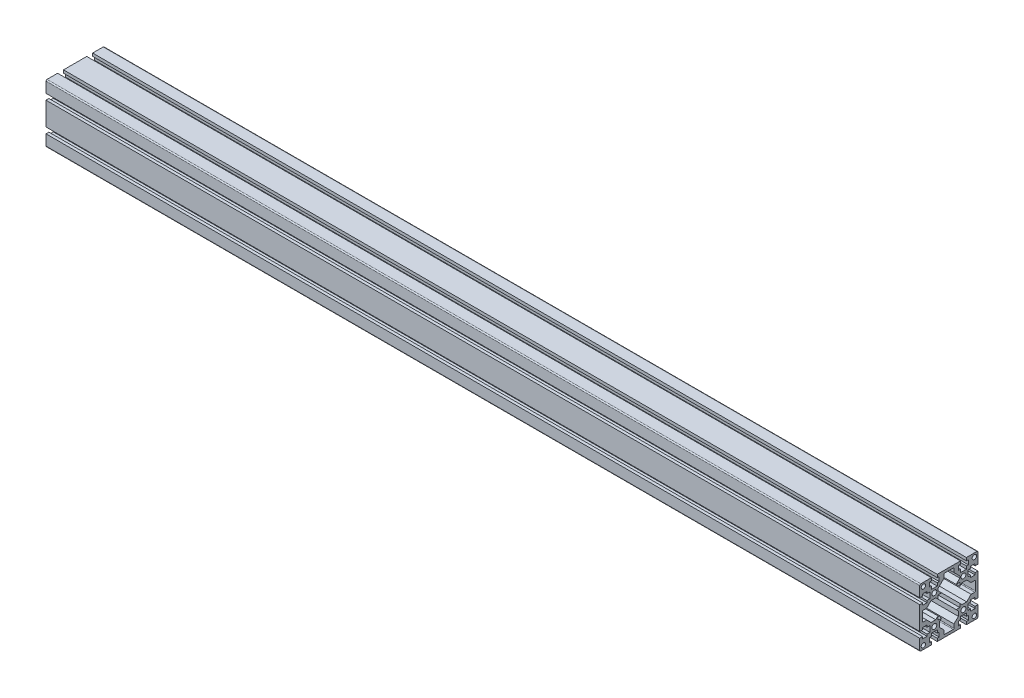
SolidWorks part; units mm, degrees
ref_plane "Front Plane" through (0, 0, 0) normal (0, 0, 1) x (1, 0, 0)
ref_plane "Top Plane" through (0, 0, 0) normal (0, 1, 0) x (1, 0, 0)
ref_plane "Right Plane" through (0, 0, 0) normal (1, 0, 0) x (0, 0, -1)
sketch "草图1" plane through (0, 0, 0) normal (0, 0, 1) x (1, 0, 0)
  line L0 (-530.3448, 0) -> (669.6552, 0)
  dimension "D1" = 1200
other "Aluminum profile 80 X 80G X R1.5(1)"
ref_plane "Plane2" through (-530.3448, 0, 0) normal (1, 0, 0) x (0, 1, 0)
sketch "Sketch1" plane through (-530.3448, 0, 0) normal (1, 0, 0) x (0, 1, 0)
  line L0 (0, 40) -> (0, 0) construction
  line L1 (0, 0) -> (40, 0) construction
  line L2 (-24.05, 40) -> (-24.05, 36)
  line L3 (-38.5, 40) -> (-24.05, 40)
  line L4 (-40, 38.5) -> (-40, 24.05)
  line L5 (-38.5, -40) -> (-24.05, -40)
  line L6 (40, 38.5) -> (40, 24.05)
  line L7 (-24.05, 36) -> (-26.75, 36)
  line L8 (-26.75, 36) -> (-26.75, 30)
  line L9 (-26.75, 30) -> (-24.05, 30)
  line L10 (-24.05, 30) -> (-24.05, 26)
  line L11 (-24.05, 26) -> (-15.95, 26)
  line L12 (-15.95, 26) -> (-15.95, 30)
  line L13 (-15.95, 30) -> (-13.25, 30)
  line L14 (-13.25, 30) -> (-13.25, 36)
  line L15 (-13.25, 36) -> (-15.95, 36)
  line L16 (-15.95, 36) -> (-15.95, 40)
  line L17 (-40, 15.95) -> (-36, 15.95)
  line L18 (-36, 15.95) -> (-36, 13.25)
  line L19 (-15.95, 40) -> (15.95, 40)
  line L20 (-20, 20) -> (-20, 40) construction
  line L21 (20, 20) -> (20, 40) construction
  line L22 (15.95, 36) -> (15.95, 40)
  line L23 (13.25, 36) -> (15.95, 36)
  line L24 (13.25, 30) -> (13.25, 36)
  line L25 (15.95, 30) -> (13.25, 30)
  line L26 (-36, 13.25) -> (-30, 13.25)
  line L27 (-30, 13.25) -> (-30, 15.95)
  line L28 (-26, 15.95) -> (-26, 24.05)
  line L29 (-26, 24.05) -> (-30, 24.05)
  line L30 (-30, 24.05) -> (-30, 26.75)
  line L31 (-30, 26.75) -> (-36, 26.75)
  line L32 (-36, 26.75) -> (-36, 24.05)
  line L33 (-36, 24.05) -> (-40, 24.05)
  line L34 (-30, 15.95) -> (-26, 15.95)
  line L35 (15.95, 26) -> (15.95, 30)
  line L36 (24.05, 26) -> (15.95, 26)
  line L37 (24.05, 30) -> (24.05, 26)
  line L38 (26.75, 30) -> (24.05, 30)
  line L39 (26.75, 36) -> (26.75, 30)
  line L40 (24.05, 36) -> (26.75, 36)
  line L41 (24.05, 40) -> (24.05, 36)
  line L42 (24.05, -40) -> (24.05, -36)
  line L43 (24.05, -36) -> (26.75, -36)
  line L44 (26.75, -36) -> (26.75, -30)
  line L45 (26.75, -30) -> (24.05, -30)
  line L46 (24.05, -30) -> (24.05, -26)
  line L47 (24.05, -26) -> (15.95, -26)
  line L48 (15.95, -26) -> (15.95, -30)
  line L49 (15.95, -30) -> (13.25, -30)
  line L50 (13.25, -30) -> (13.25, -36)
  line L51 (13.25, -36) -> (15.95, -36)
  line L52 (15.95, -36) -> (15.95, -40)
  line L53 (-15.95, -36) -> (-15.95, -40)
  line L54 (-13.25, -36) -> (-15.95, -36)
  line L55 (-13.25, -30) -> (-13.25, -36)
  line L56 (-15.95, -30) -> (-13.25, -30)
  line L57 (-15.95, -26) -> (-15.95, -30)
  line L58 (-24.05, -26) -> (-15.95, -26)
  line L59 (-24.05, -30) -> (-24.05, -26)
  line L60 (-26.75, -30) -> (-24.05, -30)
  line L61 (-26.75, -36) -> (-26.75, -30)
  line L62 (-24.05, -36) -> (-26.75, -36)
  line L63 (-24.05, -40) -> (-24.05, -36)
  line L64 (-30, -15.95) -> (-26, -15.95)
  line L65 (-36, -26.75) -> (-36, -24.05)
  line L66 (-30, -26.75) -> (-36, -26.75)
  line L67 (-30, -24.05) -> (-30, -26.75)
  line L68 (-26, -24.05) -> (-30, -24.05)
  line L69 (-26, -15.95) -> (-26, -24.05)
  line L70 (-30, -13.25) -> (-30, -15.95)
  line L71 (-36, -13.25) -> (-30, -13.25)
  line L72 (-36, -15.95) -> (-36, -13.25)
  line L73 (36, 24.05) -> (40, 24.05)
  line L74 (40, 15.95) -> (36, 15.95)
  line L75 (36, -15.95) -> (36, -13.25)
  line L76 (36, -13.25) -> (30, -13.25)
  line L77 (30, -13.25) -> (30, -15.95)
  line L78 (26, -15.95) -> (26, -24.05)
  line L79 (26, -24.05) -> (30, -24.05)
  line L80 (30, -24.05) -> (30, -26.75)
  line L81 (30, -26.75) -> (36, -26.75)
  line L82 (36, -26.75) -> (36, -24.05)
  line L83 (30, -15.95) -> (26, -15.95)
  line L84 (30, 15.95) -> (26, 15.95)
  line L85 (36, 26.75) -> (36, 24.05)
  line L86 (30, 26.75) -> (36, 26.75)
  line L87 (30, 24.05) -> (30, 26.75)
  line L88 (26, 24.05) -> (30, 24.05)
  line L89 (26, 15.95) -> (26, 24.05)
  line L90 (30, 13.25) -> (30, 15.95)
  line L91 (36, 13.25) -> (30, 13.25)
  line L92 (36, 15.95) -> (36, 13.25)
  line L93 (-36, -15.95) -> (-40, -15.95)
  line L94 (-36, -24.05) -> (-40, -24.05)
  line L95 (36, -15.95) -> (40, -15.95)
  line L96 (36, -24.05) -> (40, -24.05)
  line L97 (-13, 18) -> (-10, 15)
  line L98 (-15, 15) -> (-10, 15)
  line L99 (-15, 15) -> (-15, 10)
  line L100 (-15, -15) -> (-10, -15)
  line L101 (15, 15) -> (15, 10)
  line L102 (-18, 13) -> (-15, 10)
  line L104 (13, 18) -> (10, 15)
  line L105 (13, -18) -> (10, -15)
  line L106 (20, -15) -> (15, -10)
  line L107 (-18, -13) -> (-15, -10)
  line L108 (-13, -18) -> (-10, -15)
  line L109 (15, -10) -> (15, -15)
  line L110 (10, 15) -> (15, 15)
  line L111 (-15, -10) -> (-15, -15)
  line L112 (10, -15) -> (15, -15)
  line L113 (15, 10) -> (20, 15)
  line L235 (24.05, 40) -> (38.5, 40)
  line L249 (-40, 15.95) -> (-40, -15.95)
  line L250 (-20, 20) -> (-26, 20) construction
  line L264 (40, 15.95) -> (40, -15.95)
  line L265 (-13, 24.5) -> (-7, 30.5)
  line L266 (-7, 30.5) -> (-7, 35.5)
  line L267 (7, 35.5) -> (7, 30.5)
  line L268 (7, 30.5) -> (13, 24.5)
  line L269 (-6, -36.5) -> (6, -36.5)
  line L270 (-13, 24.5) -> (-13, 18)
  line L271 (-35.5, 7) -> (-30.5, 7)
  line L272 (-30.5, 7) -> (-24.5, 13)
  line L273 (-24.5, 13) -> (-18, 13)
  line L274 (13, 24.5) -> (13, 18)
  line L275 (-15.95, -40) -> (15.95, -40)
  line L276 (35.5, 7) -> (30.5, 7)
  line L277 (30.5, 7) -> (22.5, 15)
  line L278 (24.05, -40) -> (38.5, -40)
  line L279 (20, 15) -> (22.5, 15)
  line L333 (-13, -24.5) -> (-13, -18)
  line L336 (-13, -24.5) -> (-7, -30.5)
  line L385 (-7, -30.5) -> (-7, -35.5)
  line L386 (-36.5, 6) -> (-36.5, -6)
  line L387 (7, -35.5) -> (7, -30.5)
  line L429 (7, -30.5) -> (13, -24.5)
  line L430 (13, -24.5) -> (13, -18)
  line L494 (20, -15) -> (22.5, -15)
  line L496 (30.5, -7) -> (22.5, -15)
  line L497 (35.5, -7) -> (30.5, -7)
  line L498 (-24.5, -13) -> (-18, -13)
  line L499 (-30.5, -7) -> (-24.5, -13)
  line L500 (-35.5, -7) -> (-30.5, -7)
  line L512 (40, -24.05) -> (40, -38.5)
  line L519 (-40, -24.05) -> (-40, -38.5)
  line L520 (-6, 36.5) -> (6, 36.5)
  line L523 (36.5, 6) -> (36.5, -6)
  circle A0 centre (-20, 20) radius 3.4
  circle A2 centre (20, 20) radius 3.4
  circle A3 centre (20, -20) radius 3.4
  circle A7 centre (-20, -20) radius 3.4
  arc A8 (-38.5, 40) -> (-40, 38.5) centre (-38.5, 38.5) ccw
  arc A9 (-40, -38.5) -> (-38.5, -40) centre (-38.5, -38.5) ccw
  arc A10 (38.5, -40) -> (40, -38.5) centre (38.5, -38.5) ccw
  arc A11 (38.5, 40) -> (40, 38.5) centre (38.5, 38.5) cw
  circle A12 centre (-35, 35) radius 3
  circle A13 centre (35, 35) radius 3
  circle A14 centre (35, -35) radius 3
  arc A15 (-6, 36.5) -> (-7, 35.5) centre (-6, 35.5) ccw
  arc A16 (6, 36.5) -> (7, 35.5) centre (6, 35.5) cw
  arc A17 (-36.5, 6) -> (-35.5, 7) centre (-35.5, 6) cw
  arc A18 (-36.5, -6) -> (-35.5, -7) centre (-35.5, -6) ccw
  arc A19 (36.5, -6) -> (35.5, -7) centre (35.5, -6) cw
  arc A20 (36.5, 6) -> (35.5, 7) centre (35.5, 6) ccw
  arc A21 (6, -36.5) -> (7, -35.5) centre (6, -35.5) ccw
  arc A22 (-6, -36.5) -> (-7, -35.5) centre (-6, -35.5) cw
  point P48 (-20, 20)
  point P97 (0, 0)
  point P104 (-7, 36.5)
  point P185 (40, 40)
  point P187 (40, -40)
  point P188 (-40, -40)
  point P190 (-40, 40)
  dimension "D1" = 80
  dimension "D2" = 80
  dimension "D3" = 20
  dimension "D4" = 8.1
  dimension "D5" = 45
  dimension "D6" = 7
  dimension "D7" = 13.5
  dimension "D8" = 6
  dimension "D12" = 5
  dimension "D13" = 5
  dimension "D14" = 20
  dimension "D18" = 1
  dimension "D19" = 14
  dimension "D15" = 6.8
  dimension "D27" = 45
  dimension "D20" = 1.5
  dimension "D11" = 6
  dimension "D9" = 4
  dimension "D10" = 14
  dimension "D16" = 14
  dimension "D17" = 45
  dimension "D21" = 3.5
  dimension "D22" = 3.5
  dimension "D23" = 73
  dimension "D24" = 30
  dimension "D25" = 30
  dimension "D26" = 45
  dimension "D28" = 5
sketch "Sketch10" plane through (669.6552, 0, 0) normal (1, 0, 0) x (0, 0, -1)
  circle A0 centre (35, -35) radius 3
  circle A1 centre (-35, -35) radius 3 construction
  circle A2 centre (35, 35) radius 3 construction
  dimension "D1" = 6
  dimension "D2" = 70
  dimension "D3" = 70
extrude "Cut-Extrude1" cut sketch "Sketch10" against normal through all
